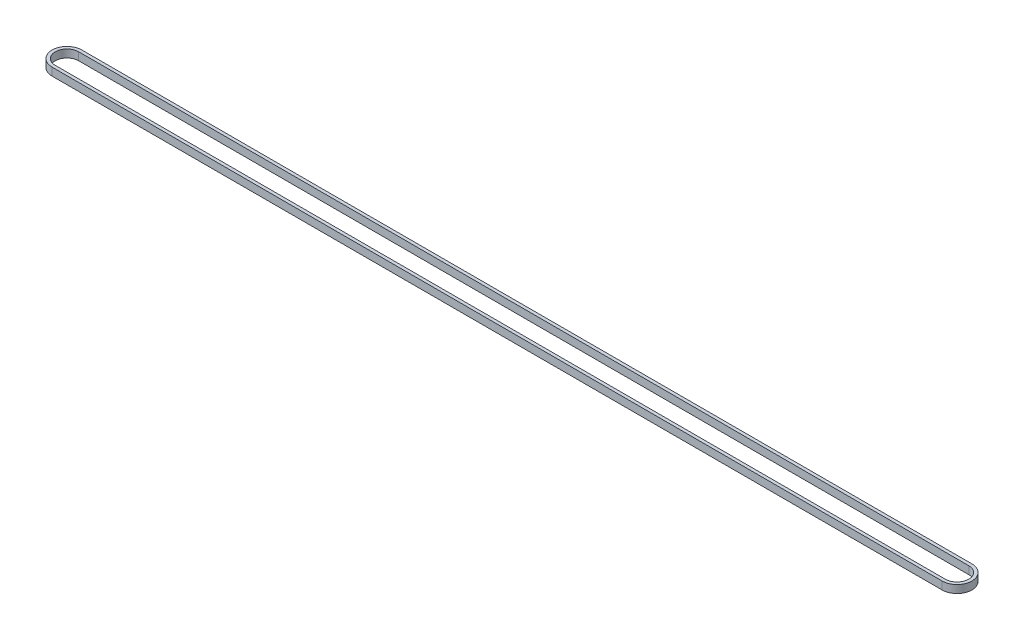
SolidWorks part; units mm, degrees
ref_plane "Front Plane" through (0, 0, 0) normal (0, 0, 1) x (1, 0, 0)
ref_plane "Top Plane" through (0, 0, 0) normal (0, 1, 0) x (1, 0, 0)
ref_plane "Right Plane" through (0, 0, 0) normal (1, 0, 0) x (0, 0, -1)
sketch "Sketch1" plane through (0, 0, 0) normal (0, 1, 0) x (1, 0, 0)
  line L0 (284.5, 0) -> (-284.5, 0) construction
  line L1 (284.5, -7.5) -> (-284.5, -7.5)
  line L2 (284.5, 7.5) -> (-284.5, 7.5)
  line L3 (284.5, -9.5) -> (-284.5, -9.5)
  line L4 (284.5, 9.5) -> (-284.5, 9.5)
  arc A0 (284.5, -7.5) -> (284.5, 7.5) centre (284.5, 0) ccw
  arc A1 (-284.5, 7.5) -> (-284.5, -7.5) centre (-284.5, 0) ccw
  arc A2 (-284.5, 9.5) -> (-284.5, -9.5) centre (-284.5, 0) ccw
  arc A3 (284.5, -9.5) -> (284.5, 9.5) centre (284.5, 0) ccw
  point P2 (0, 0)
  dimension "D2" = 7.5
  dimension "D3" = 569
  dimension "D1" = 2
extrude "Boss-Extrude1" add sketch "Sketch1" along normal blind 5
